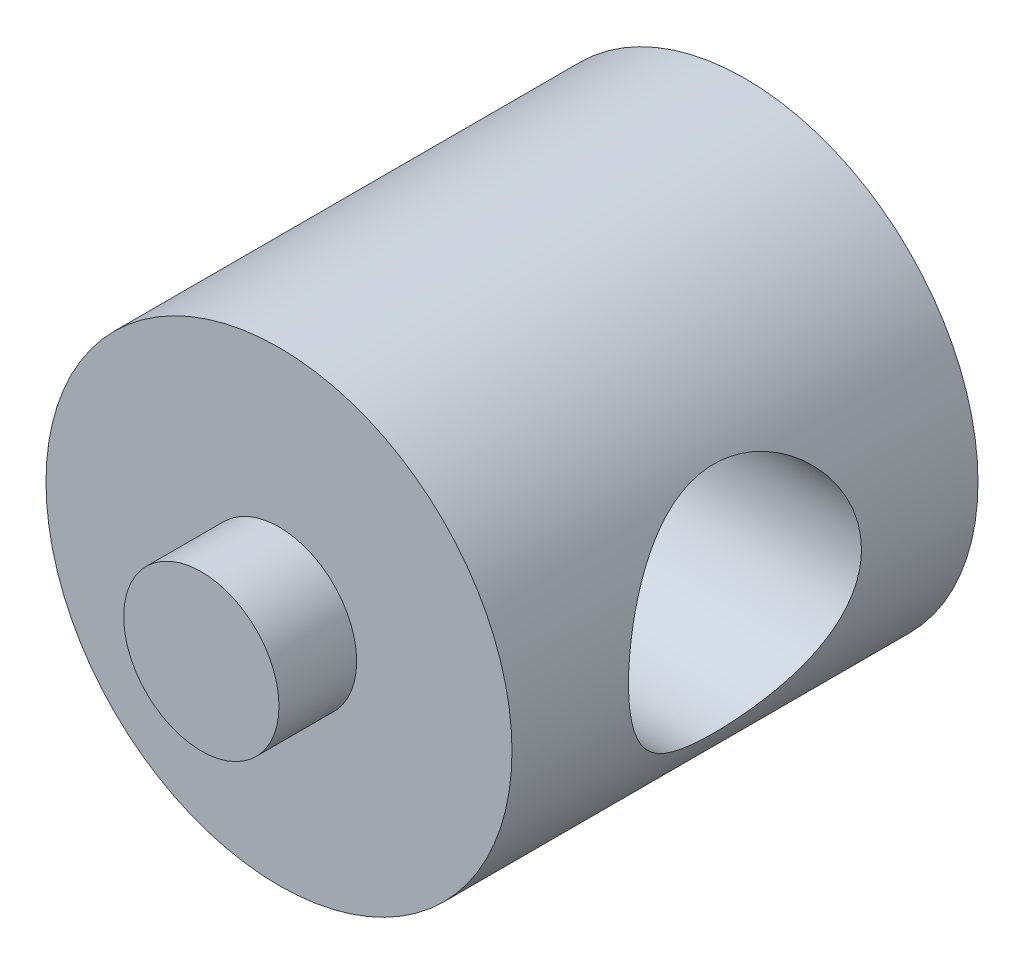
from build123d import *

# Parameters (mm, degrees)
BOSS_EXTRUDE1_DEPTH      = 9.525
BOSS_EXTRUDE1_DEPTH_BACK = 9.525
SKETCH1_R                = 9.525
BOSS_EXTRUDE2_DEPTH      = 12.7
BOSS_EXTRUDE2_DEPTH_BACK = 12.7
BOSS_EXTRUDE2_START      = -9.525
SKETCH2_R                = 3.175
CUT_EXTRUDE1_DEPTH       = 19.513272266
CUT_EXTRUDE1_DEPTH_BACK  = 19.513272266
SKETCH3_R                = 4.7625


with BuildPart() as part:
    # Sketch1 → Boss-Extrude1 (new, two sides: drawn at the far end of the back side and taken through both)
    with BuildSketch(Plane.XY.offset(-BOSS_EXTRUDE1_DEPTH_BACK)):
        Circle(SKETCH1_R)
    extrude(amount=BOSS_EXTRUDE1_DEPTH + BOSS_EXTRUDE1_DEPTH_BACK)

    # Sketch2 → Boss-Extrude2 (add, two sides: drawn at the far end of the back side and taken through both)
    with BuildSketch(Plane.XY.offset(9.525).offset(BOSS_EXTRUDE2_START - BOSS_EXTRUDE2_DEPTH_BACK)):
        Circle(SKETCH2_R)
    extrude(amount=BOSS_EXTRUDE2_DEPTH + BOSS_EXTRUDE2_DEPTH_BACK)

    # Sketch3 → Cut-Extrude1 (cut, two sides: drawn at the far end of the back side and taken through both)
    with BuildSketch(Plane(origin=(0, 0, 0), x_dir=(0, 0, -1), z_dir=(1, 0, 0)).offset(-CUT_EXTRUDE1_DEPTH_BACK)):
        Circle(SKETCH3_R)
    extrude(amount=CUT_EXTRUDE1_DEPTH + CUT_EXTRUDE1_DEPTH_BACK, mode=Mode.SUBTRACT)


solid = part.part
